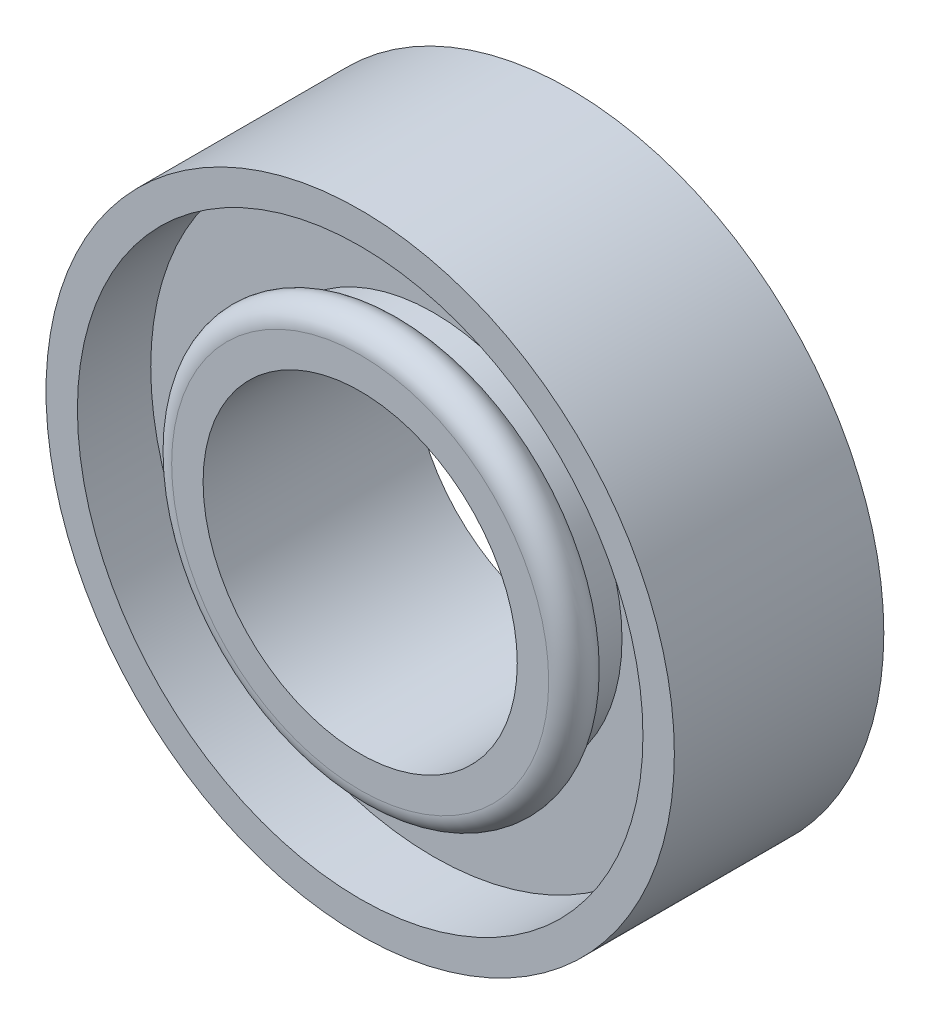
from build123d import *


with BuildPart() as part:
    # 草图1 → 旋转2 (revolve)
    with BuildSketch(Plane(origin=(0, 0, 0), x_dir=(0, 0, -1), z_dir=(1, 0, 0)), mode=Mode.PRIVATE) as revolve_2_sk:
        with BuildLine():
            Line((0, 15), (0, 7.5))
            Line((0, 7.5), (5, 7.5))
            Line((5, 7.5), (5, 9))
            ThreePointArc((5, 9), (4, 10), (3, 9))
            Line((3, 9), (1.5, 9))
            Line((1.5, 9), (1.5, 13.5))
            Line((1.5, 13.5), (5, 13.5))
            Line((5, 13.5), (5, 15))
            Line((5, 15), (0, 15))
        make_face()
    revolve_2 = revolve(revolve_2_sk.sketch.rotate(Axis((0, 0, 4.217424625), (0, 0, -1)), 90), axis=Axis((0, 0, 4.217424625), (0, 0, -1)))

    # 镜向2: 旋转2 across plane
    add(revolve_2.mirror(Plane(origin=(0, 15, 0), x_dir=(1, 0, 0), z_dir=(0, 0, -1))))


solid = part.part
